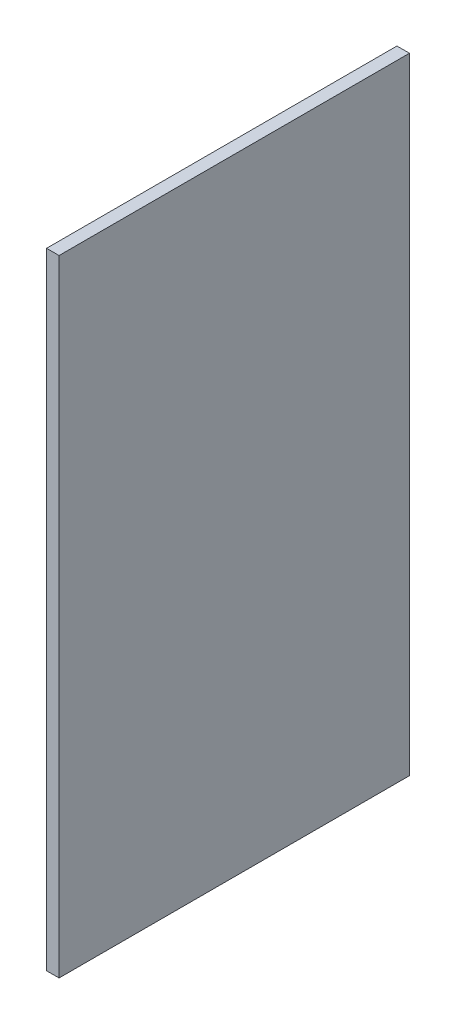
from build123d import *

# Parameters (mm, degrees)
SKETCH_1_W      = 112
SKETCH_1_H      = 200
EXTRUDE_1_DEPTH = 4


with BuildPart() as part:
    # 草图1 → 凸台-拉伸1 (new body)
    with BuildSketch(Plane(origin=(0, 0, 0), x_dir=(0, 0, -1), z_dir=(1, 0, 0))):
        with Locations((56, 100)):
            Rectangle(SKETCH_1_W, SKETCH_1_H)
    extrude(amount=EXTRUDE_1_DEPTH)


solid = part.part
